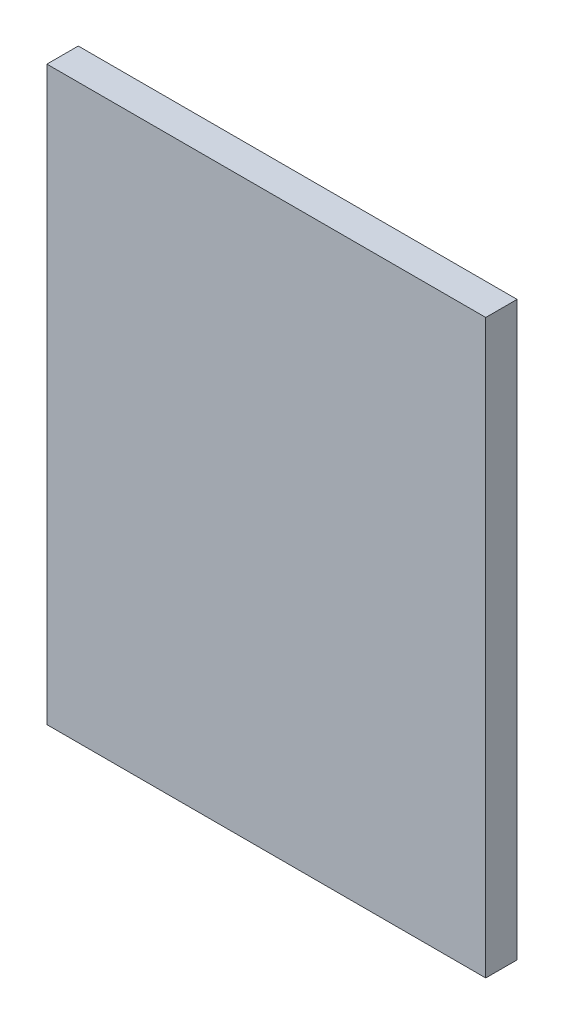
from build123d import *

# Parameters (mm, degrees)
SKETCH1_W           = 280
SKETCH1_H           = 365
BOSS_EXTRUDE1_DEPTH = 20


with BuildPart() as part:
    # Sketch1 → Boss-Extrude1 (new body)
    with BuildSketch(Plane.XY):
        with Locations((-140, 182.5)):
            Rectangle(SKETCH1_W, SKETCH1_H)
    extrude(amount=BOSS_EXTRUDE1_DEPTH)


solid = part.part
